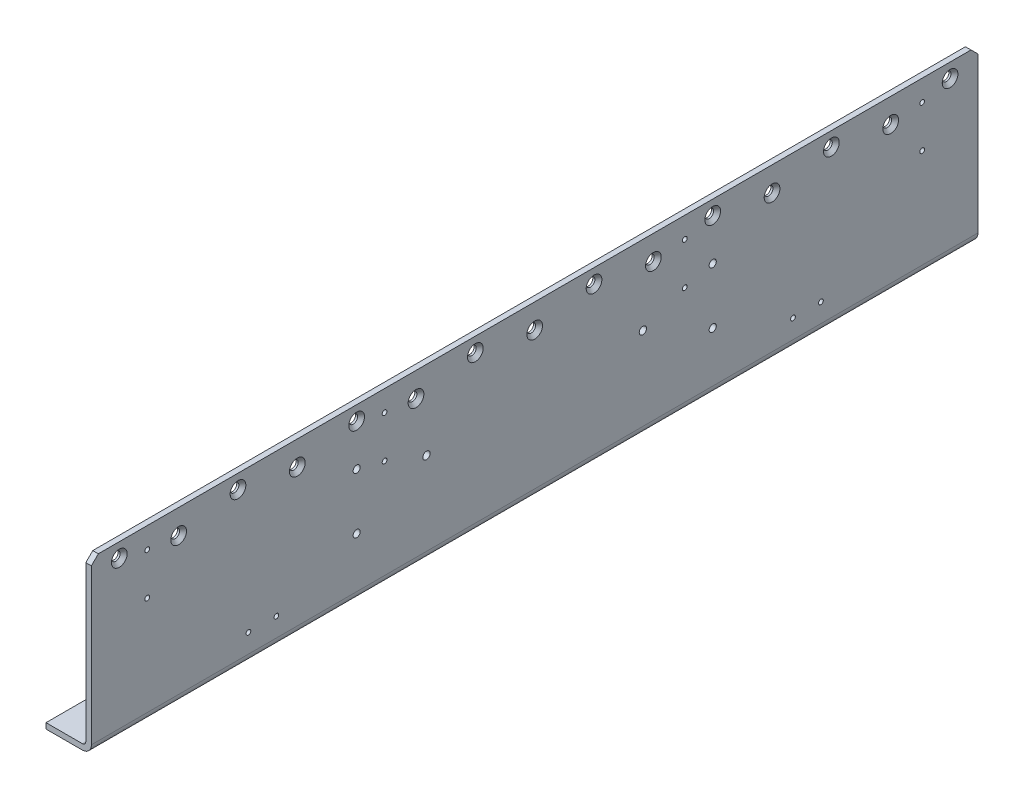
SolidWorks part; units mm, degrees
material "1023 碳钢板 (SS)"
ref_plane "Front Plane" through (0, 0, 0) normal (0, 0, 1) x (1, 0, 0)
ref_plane "Top Plane" through (0, 0, 0) normal (0, 1, 0) x (1, 0, 0)
ref_plane "Right Plane" through (0, 0, 0) normal (1, 0, 0) x (0, 0, -1)
sketch "Sketch1" plane through (0, 0, 0) normal (0, 0, 1) x (1, 0, 0)
  line L0 (0, 0) -> (0, -232)
  line L1 (-13, -245) -> (-65, -245)
  line L2 (-8, 0) -> (-8, -232)
  line L3 (-13, -237) -> (-65, -237)
  line L4 (0, 0) -> (0, -245) construction
  line L5 (0, -245) -> (-65, -245) construction
  line L6 (-8, 0) -> (-8, -237) construction
  line L7 (-8, -237) -> (-65, -237) construction
  line L8 (0, 0) -> (-8, 0)
  line L9 (-65, -237) -> (-65, -245)
  arc A0 (0, -232) -> (-13, -245) centre (-13, -232) cw
  arc A1 (-8, -232) -> (-13, -237) centre (-13, -232) cw
  point P10 (0, -245)
  dimension "D4" = 13
  dimension "D5" = 5
  dimension "D1" = 245
  dimension "D2" = 65
  dimension "D3" = 8
extrude "Boss-Extrude1" add sketch "Sketch1" along normal blind 1270 contours L9 L1 A0 L0 L8 L2 A1 L3
sketch "Sketch3" plane through (-8, 0, 0) normal (-1, 0, 0) x (0, 0, 1)
  line L0 (0, 0) -> (0, -232) construction
  line L1 (1270, 0) -> (0, 0) construction
  circle A0 centre (40, -20.5) radius 6.25
  circle A1 centre (210, -20.5) radius 6.25
  circle A2 centre (380, -20.5) radius 6.25
  circle A3 centre (550, -20.5) radius 6.25
  circle A4 centre (720, -20.5) radius 6.25
  circle A5 centre (890, -20.5) radius 6.25
  circle A6 centre (1060, -20.5) radius 6.25
  circle A7 centre (1230, -20.5) radius 6.25
  circle A8 centre (125, -35) radius 6.25
  circle A9 centre (295, -35) radius 6.25
  circle A10 centre (465, -35) radius 6.25
  circle A11 centre (635, -35) radius 6.25
  circle A12 centre (805, -35) radius 6.25
  circle A13 centre (975, -35) radius 6.25
  circle A14 centre (1145, -35) radius 6.25
  dimension "D1" = 40
  dimension "D2" = 12.5
  dimension "D3" = 20.5
  dimension "D5" = 12.5
  dimension "D6" = 85
  dimension "D7" = 14.5
  dimension "D4" = 8
  dimension "D8" = 7
extrude "Cut-Extrude1" cut sketch "Sketch3" against normal blind 3
sketch "Sketch4" plane through (-5, 0, 0) normal (-1, 0, 0) x (0, 0, 1)
  circle A0 centre (1230, -20.5) radius 6.25 construction
  circle A1 centre (1145, -35) radius 6.25 construction
  circle A2 centre (1060, -20.5) radius 6.25 construction
  circle A3 centre (975, -35) radius 6.25 construction
  circle A4 centre (890, -20.5) radius 6.25 construction
  circle A5 centre (635, -35) radius 6.25 construction
  circle A6 centre (550, -20.5) radius 6.25 construction
  circle A7 centre (465, -35) radius 6.25 construction
  circle A8 centre (380, -20.5) radius 6.25 construction
  circle A9 centre (295, -35) radius 6.25 construction
  circle A10 centre (210, -20.5) radius 6.25 construction
  circle A11 centre (125, -35) radius 6.25 construction
  circle A12 centre (40, -20.5) radius 6.25 construction
  circle A13 centre (1230, -20.5) radius 6.25
  circle A14 centre (1145, -35) radius 6.25
  circle A15 centre (1060, -20.5) radius 6.25
  circle A16 centre (975, -35) radius 6.25
  circle A17 centre (890, -20.5) radius 6.25
  circle A18 centre (635, -35) radius 6.25
  circle A19 centre (550, -20.5) radius 6.25
  circle A20 centre (465, -35) radius 6.25
  circle A21 centre (380, -20.5) radius 6.25
  circle A22 centre (295, -35) radius 6.25
  circle A23 centre (210, -20.5) radius 6.25
  circle A24 centre (125, -35) radius 6.25
  circle A25 centre (40, -20.5) radius 6.25
  circle A26 centre (805, -35) radius 6.25 construction
  circle A27 centre (720, -20.5) radius 6.25 construction
  circle A28 centre (805, -35) radius 6.25
  circle A29 centre (720, -20.5) radius 6.25
extrude "Cut-Extrude2" cut sketch "Sketch4" against normal blind 5 draft 45 draft outward yes
sketch "Sketch5" plane through (0, 0, 0) normal (1, 0, 0) x (0, 0, -1)
  line L0 (-1270, -245) -> (0, -245) construction
  line L1 (-1270, 0) -> (-1270, -232) construction
  line L2 (-635, 0) -> (-635, -166.9356) construction
  line L3 (-1270, 0) -> (0, 0) construction
  circle A0 centre (-1190, -30) radius 3
  circle A1 centre (-1190, -90) radius 3
  circle A2 centre (-1045, -205) radius 3
  circle A3 centre (-1005, -205) radius 3
  circle A4 centre (-850, -30) radius 3
  circle A5 centre (-850, -90) radius 3
  circle A6 centre (-890, -80) radius 5
  circle A7 centre (-890, -160) radius 5
  circle A8 centre (-790, -113) radius 5.25
  circle A11 centre (-480, -113) radius 5.25
  circle A12 centre (-265, -205) radius 3
  circle A13 centre (-225, -205) radius 3
  circle A14 centre (-420, -30) radius 3
  circle A15 centre (-420, -90) radius 3
  circle A16 centre (-380, -80) radius 5
  circle A17 centre (-380, -160) radius 5
  circle A18 centre (-80, -90) radius 3
  circle A19 centre (-80, -30) radius 3
  dimension "D9" = 10.5
  dimension "D12" = 6
  dimension "D14" = 10
  dimension "D15" = 225
  dimension "D1" = 60
  dimension "D2" = 155
  dimension "D3" = 340
  dimension "D4" = 40
  dimension "D5" = 80
  dimension "D6" = 85
  dimension "D7" = 45
  dimension "D8" = 33
  dimension "D10" = 115
  dimension "D11" = 100
  dimension "D13" = 80
extrude "Cut-Extrude3" cut sketch "Sketch5" against normal blind 8
hole_wizard "M12 Tapped Hole1" positions "Sketch6" profile "Sketch7" tap size "M12" standard "ISO"
sketch "Sketch6" plane through (0, 0, 0) normal (1, 0, 0) x (0, 0, -1)
  point P0 (-890, -80)
  point P3 (-890, -160)
  point P6 (-380, -80)
  point P9 (-380, -160)
sketch "Sketch7" plane through (0, -80, 890) normal (0, 1, 0) x (0, 0, -1)
  line L0 (0, 0) -> (0, 28.3144)
  line L1 (0, 28.3144) -> (5.1, 25.25)
  line L2 (5.1, 25.25) -> (5.1, 0)
  line L5 (5.1, 0) -> (0, 0)
  line L10 (0, 28.3144) -> (-5.1, 25.25) construction
  line L11 (0, -6.35) -> (0, 107.95) construction
  dimension "螺纹孔钻头直径" = 10.2
  dimension "螺纹孔钻头深度" = 25.25
  dimension "导头角度" = 118
cosmetic thread "Hole Thread Line1" parameters "D1"=20, "D2"=12
cosmetic thread "Hole Thread Line2" parameters "D1"=20, "D2"=12
cosmetic thread "Hole Thread Line3" parameters "D1"=20, "D2"=12
cosmetic thread "Hole Thread Line4" parameters "D1"=20, "D2"=12
hole_wizard "M8 Tapped Hole1" positions "Sketch8" profile "Sketch9" tap size "M8" standard "ISO"
sketch "Sketch8" plane through (0, 0, 0) normal (1, 0, 0) x (0, 0, -1)
  point P0 (-1190, -30)
  point P3 (-1190, -90)
  point P6 (-1045, -205)
  point P9 (-1005, -205)
  point P12 (-850, -90)
  point P15 (-850, -30)
  point P18 (-420, -90)
  point P21 (-420, -30)
  point P24 (-265, -205)
  point P27 (-225, -205)
  point P30 (-80, -90)
  point P33 (-80, -30)
sketch "Sketch9" plane through (0, -30, 1190) normal (0, 1, 0) x (0, 0, -1)
  line L0 (0, 0) -> (0, 21.7929)
  line L1 (0, 21.7929) -> (3.4, 19.75)
  line L2 (3.4, 19.75) -> (3.4, 0)
  line L5 (3.4, 0) -> (0, 0)
  line L10 (0, 21.7929) -> (-3.4, 19.75) construction
  line L11 (0, -6.35) -> (0, 107.95) construction
  dimension "螺纹孔钻头直径" = 6.8
  dimension "螺纹孔钻头深度" = 19.75
  dimension "导头角度" = 118
cosmetic thread "Hole Thread Line5" parameters "D1"=16, "D2"=8
cosmetic thread "Hole Thread Line6" parameters "D1"=16, "D2"=8
cosmetic thread "Hole Thread Line7" parameters "D1"=16, "D2"=8
cosmetic thread "Hole Thread Line8" parameters "D1"=16, "D2"=8
cosmetic thread "Hole Thread Line9" parameters "D1"=16, "D2"=8
cosmetic thread "Hole Thread Line10" parameters "D1"=16, "D2"=8
cosmetic thread "Hole Thread Line11" parameters "D1"=16, "D2"=8
cosmetic thread "Hole Thread Line12" parameters "D1"=16, "D2"=8
cosmetic thread "Hole Thread Line13" parameters "D1"=16, "D2"=8
cosmetic thread "Hole Thread Line14" parameters "D1"=16, "D2"=8
cosmetic thread "Hole Thread Line15" parameters "D1"=16, "D2"=8
cosmetic thread "Hole Thread Line16" parameters "D1"=16, "D2"=8
chamfer "Chamfer1" distance 10 angle 45 2 edges at (-4, 0, 0) (-4, 0, 1270)
sketch "Sketch10" plane through (0, -237, 0) normal (0, 1, 0) x (1, 0, 0)
  line L1 (-13, -1270) -> (-65, -1270) construction
  line L2 (-13, 0) -> (-65, 0) construction
  line L3 (-65, -1270) -> (-65, 0) construction
  line L4 (0, -1260) -> (0, -10) construction
  circle A0 centre (-40, -890) radius 6.5
  circle A1 centre (-40, -380) radius 6.5
  circle A2 centre (-40, -537.5) radius 6.5
  circle A3 centre (-40, -732.5) radius 6.5
  circle A4 centre (-40, -635) radius 7.5
  point P15 (-65, -635)
  dimension "D3" = 13
  dimension "D4" = 195
  dimension "D8" = 15
  dimension "D1" = 380
  dimension "D2" = 380
  dimension "D5" = 97.5
  dimension "D6" = 40
  dimension "D7" = 97.5
extrude "Cut-Extrude4" cut sketch "Sketch10" against normal blind 8
